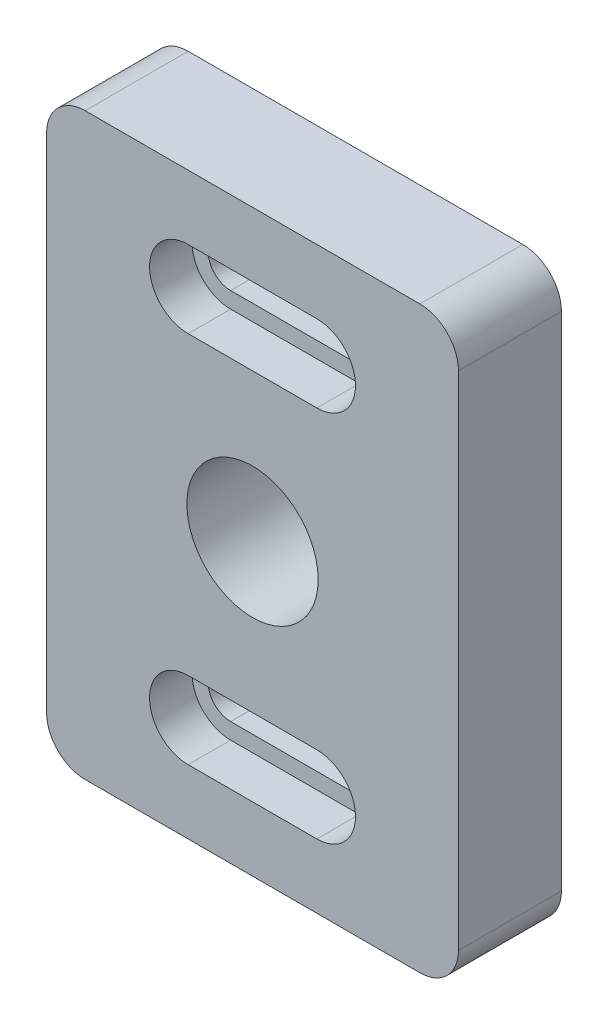
from build123d import *

# Parameters (mm, degrees)
SKETCH1_W           = 32
SKETCH1_H           = 45
BOSS_EXTRUDE1_DEPTH = 8
M12_TAPPED_HOLE1_D  = 10.2
CUT_EXTRUDE1_DEPTH  = 29.744564704
CUT_EXTRUDE2_DEPTH  = 3.3
FILLET1_R           = 3


with BuildPart() as part:
    # Sketch1 → Boss-Extrude1 (new body)
    with BuildSketch(Plane.XY):
        Rectangle(SKETCH1_W, SKETCH1_H)
    extrude(amount=BOSS_EXTRUDE1_DEPTH)

    # M12 Tapped Hole1 (through all)
    with Locations(Plane.XY.offset(8)):
        with Locations((0, 0)):
            Hole(M12_TAPPED_HOLE1_D / 2)

    # Sketch5 → Cut-Extrude1 (cut, through all)
    with BuildSketch(Plane.XY.offset(8)):
        with BuildLine():
            Line((-5, -12.75), (5, -12.75))
            ThreePointArc((5, -12.75), (6.75, -14.5), (5, -16.25))
            Line((5, -16.25), (-5, -16.25))
            ThreePointArc((-5, -16.25), (-6.75, -14.5), (-5, -12.75))
        make_face()
        with BuildLine():
            Line((-5, 16.25), (5, 16.25))
            ThreePointArc((5, 16.25), (6.75, 14.5), (5, 12.75))
            Line((5, 12.75), (-5, 12.75))
            ThreePointArc((-5, 12.75), (-6.75, 14.5), (-5, 16.25))
        make_face()
    extrude(amount=-CUT_EXTRUDE1_DEPTH, mode=Mode.SUBTRACT)

    # Sketch6 → Cut-Extrude2 (cut)
    with BuildSketch(Plane.XY.offset(8)):
        with BuildLine():
            Line((-5, -11.5), (5, -11.5))
            ThreePointArc((5, -11.5), (8, -14.5), (5, -17.5))
            Line((5, -17.5), (-5, -17.5))
            ThreePointArc((-5, -17.5), (-8, -14.5), (-5, -11.5))
        make_face()
        with BuildLine():
            Line((-5, 17.5), (5, 17.5))
            ThreePointArc((5, 17.5), (8, 14.5), (5, 11.5))
            Line((5, 11.5), (-5, 11.5))
            ThreePointArc((-5, 11.5), (-8, 14.5), (-5, 17.5))
        make_face()
    extrude(amount=-CUT_EXTRUDE2_DEPTH, mode=Mode.SUBTRACT)

    # Fillet1
    fillet1_edges = [part.edges().sort_by_distance(p)[0] for p in [
        (-16, 22.5, 4),
        (16, 22.5, 4),
        (16, -22.5, 4),
        (-16, -22.5, 4),
    ]]
    fillet(fillet1_edges, radius=FILLET1_R)


solid = part.part
